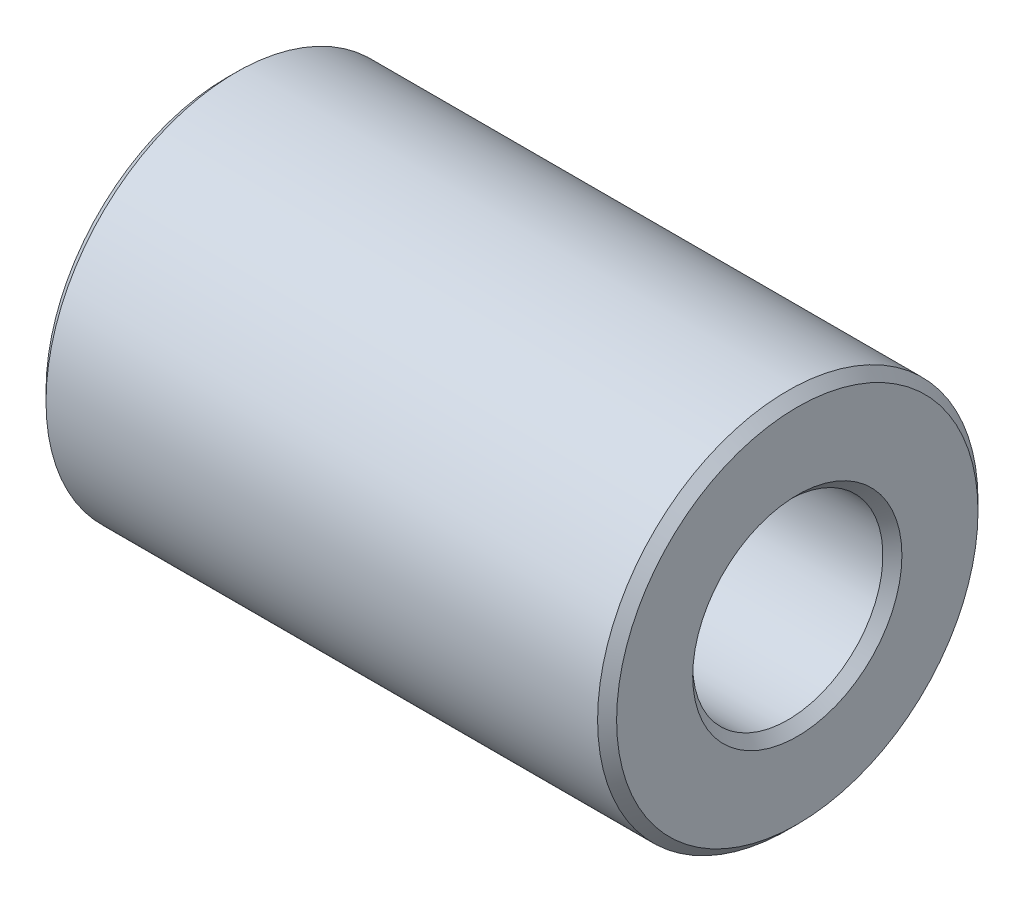
from build123d import *

# Parameters (mm, degrees)
CHAMFER1_SIZE = 0.2


with BuildPart() as part:
    # Sketch1 → Revolve1 (revolve)
    with BuildSketch(Plane.XY, mode=Mode.PRIVATE) as revolve1_sk:
        Polygon((0, 3.7), (0, 2), (12, 2), (12, 3.7), (12, 4), (11.7, 4), (0.3, 4), (0, 4), align=None)
    revolve(revolve1_sk.sketch.rotate(Axis((12, 0, 0), (-1, 0, 0)), 270), axis=Axis((12, 0, 0), (-1, 0, 0)))

    # Chamfer1
    chamfer1_edges = [part.edges().sort_by_distance(p)[0] for p in [
        (0, 0, -4),
        (12, 0, -4),
        (12, 0, -2),
        (0, 0, -2),
    ]]
    chamfer(chamfer1_edges, length=CHAMFER1_SIZE)


solid = part.part
